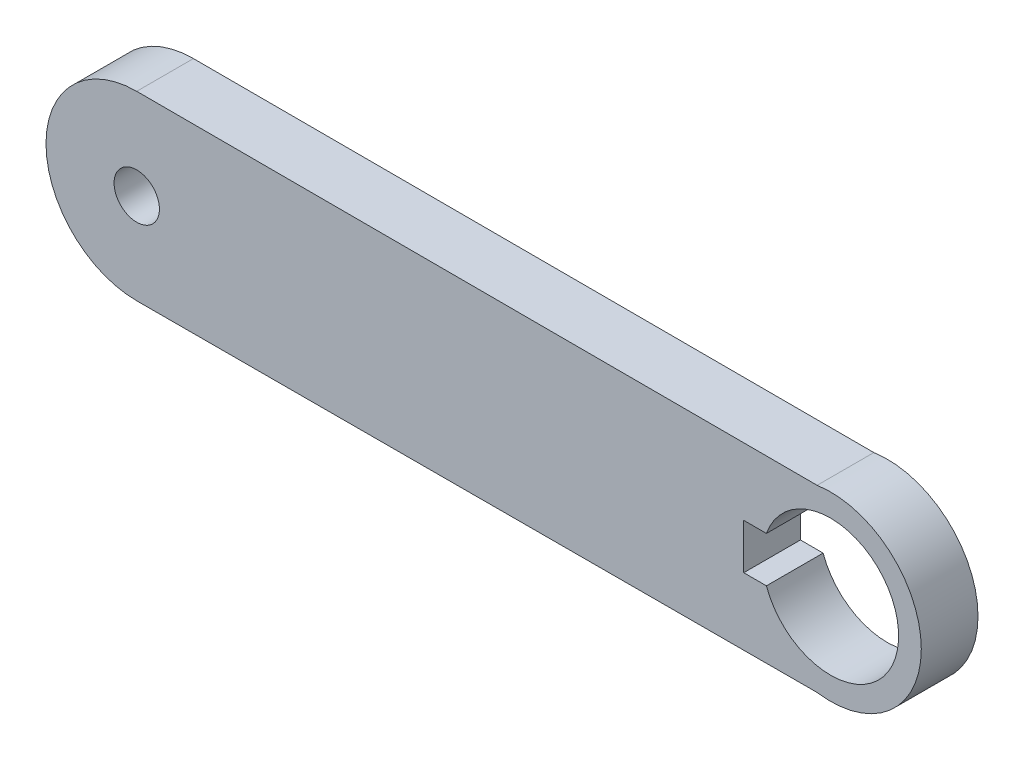
SolidWorks part; units mm, degrees
ref_plane "前视基准面" through (0, 0, 0) normal (0, 0, 1) x (1, 0, 0)
ref_plane "上视基准面" through (0, 0, 0) normal (0, 1, 0) x (1, 0, 0)
ref_plane "右视基准面" through (0, 0, 0) normal (1, 0, 0) x (0, 0, -1)
other "Configuration Table"
sketch "草图1" plane through (0, 0, 0) normal (0, 0, 1) x (1, 0, 0)
  line L0 (-72.9972, -0.2687) -> (74.0561, -0.2687) construction
  line L1 (-53.7308, 24.699) -> (-53.7308, -29.5614) construction
  line L2 (6.2692, 28.2377) -> (6.2692, -29.5614) construction
  line L3 (-53.7308, 7.7313) -> (6.2692, 7.6431)
  line L4 (-53.7308, -8.2687) -> (6.2692, -8.1804)
  line L5 (4.797, 1.7313) -> (4.797, -2.2687) construction
  line L6 (-0.203, 1.7313) -> (-0.203, -2.2687)
  line L7 (1.797, 1.7313) -> (-0.203, 1.7313)
  line L8 (1.797, -2.2687) -> (-0.203, -2.2687)
  arc A0 (-53.7308, 7.7313) -> (-53.7308, -8.2687) centre (-53.7308, -0.2687) ccw
  arc A1 (6.2692, -8.1804) -> (6.2692, 7.6431) centre (7.4539, -0.2687) ccw
  circle A2 centre (-53.7308, -0.2687) radius 2
  arc A3 (1.797, -2.2687) -> (1.797, 1.7313) centre (7.4539, -0.2687) ccw
  point P18 (1.797, 1.7313)
  dimension "D2" = 16
  dimension "D3" = 16
  dimension "D4" = 4
  dimension "D1" = 60
  dimension "D5" = 4
  dimension "D6" = 2
extrude "凸台-拉伸1" add sketch "草图1" along normal blind 5
